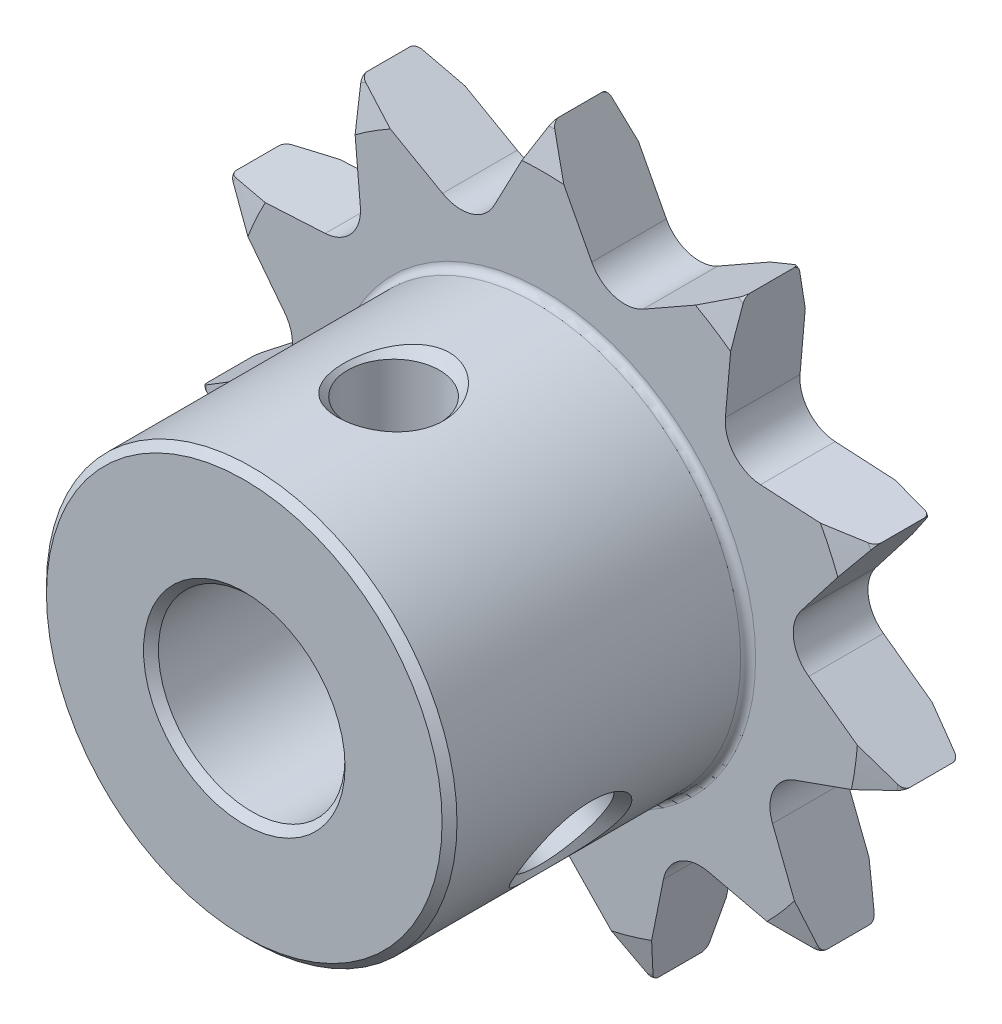
from build123d import *

# Parameters (mm, degrees)
SKETCH_2_W          = 302.005499825
SKETCH_2_H          = 246.129864536
CUT_EXTRUDE_1_DEPTH = 2


with BuildPart() as part:
    # 草图1 → 旋转1 (revolve)
    with BuildSketch(Plane(origin=(0, 0, 0), x_dir=(0, 0, -1), z_dir=(1, 0, 0)), mode=Mode.PRIVATE) as revolve_1_sk:
        with BuildLine():
            Line((-10, 2.7), (-9.8, 2.5))
            Line((-9.8, 2.5), (-0.2, 2.5))
            Line((-0.2, 2.5), (0, 2.7))
            Line((0, 2.7), (0, 8.45))
            Line((0, 8.45), (-0.241626884, 9.351763809))
            ThreePointArc((-0.241626884, 9.351763809), (-0.313059764, 9.458670668), (-0.43481205, 9.5))
            Line((-0.43481205, 9.5), (-1.56518795, 9.5))
            ThreePointArc((-1.56518795, 9.5), (-1.686940236, 9.458670668), (-1.758373116, 9.351763809))
            Line((-1.758373116, 9.351763809), (-2, 8.45))
            Line((-2, 8.45), (-2, 5.7))
            ThreePointArc((-2, 5.7), (-2.058578644, 5.558578644), (-2.2, 5.5))
            Line((-2.2, 5.5), (-9.8, 5.5))
            Line((-9.8, 5.5), (-10, 5.3))
            Line((-10, 5.3), (-10, 2.7))
        make_face()
    revolve(revolve_1_sk.sketch.rotate(Axis((0, 0, 0), (0, 0, 1)), 270), axis=Axis((0, 0, 0), (0, 0, 1)))

    # 草图2 → 切除-拉伸1 (cut)
    with BuildSketch(Plane.XY):
        with Locations((0.692673165, 3.694256879)):
            Rectangle(SKETCH_2_W, SKETCH_2_H)
        with BuildLine():
            Line((-9.403303698, -1.351990964), (-6.749929888, -2.292665419))
            ThreePointArc((-6.749929888, -2.292665419), (-6.174441043, -2.819772743), (-6.152944955, -3.59988008))
            Line((-6.152944955, -3.59988008), (-7.179620956, -6.221176972))
            Line((-7.179620956, -6.221176972), (-4.438893858, -5.578000496))
            ThreePointArc((-4.438893858, -5.578000496), (-3.6697861, -5.710298635), (-3.229944571, -6.354945026))
            Line((-3.229944571, -6.354945026), (-2.67645929, -9.115183249))
            Line((-2.67645929, -9.115183249), (-0.718540392, -7.092359827))
            ThreePointArc((-0.718540392, -7.092359827), (0, -6.787845057), (0.718540392, -7.092359827))
            Line((0.718540392, -7.092359827), (2.67645929, -9.115183249))
            Line((2.67645929, -9.115183249), (3.229944571, -6.354945026))
            ThreePointArc((3.229944571, -6.354945026), (3.6697861, -5.710298635), (4.438893858, -5.578000496))
            Line((4.438893858, -5.578000496), (7.179620956, -6.221176972))
            Line((7.179620956, -6.221176972), (6.152944955, -3.59988008))
            ThreePointArc((6.152944955, -3.59988008), (6.174441043, -2.819772743), (6.749929888, -2.292665419))
            Line((6.749929888, -2.292665419), (9.403303698, -1.351990964))
            Line((9.403303698, -1.351990964), (7.12242879, 0.298121355))
            ThreePointArc((7.12242879, 0.298121355), (6.718754582, 0.966011072), (6.917910871, 1.720574729))
            Line((6.917910871, 1.720574729), (8.641503956, 3.946442624))
            Line((8.641503956, 3.946442624), (5.830591809, 4.101471366))
            ThreePointArc((5.830591809, 4.101471366), (5.129911013, 4.445093196), (4.889504032, 5.187544557))
            Line((4.889504032, 5.187544557), (5.136087766, 7.991908562))
            Line((5.136087766, 7.991908562), (2.687583126, 6.602633199))
            ThreePointArc((2.687583126, 6.602633199), (1.912356943, 6.512889638), (1.308714211, 7.007505642))
            Line((1.308714211, 7.007505642), (0, 9.5))
            Line((0, 9.5), (-1.308714211, 7.007505642))
            ThreePointArc((-1.308714211, 7.007505642), (-1.912356943, 6.512889638), (-2.687583126, 6.602633199))
            Line((-2.687583126, 6.602633199), (-5.136087766, 7.991908562))
            Line((-5.136087766, 7.991908562), (-4.889504032, 5.187544557))
            ThreePointArc((-4.889504032, 5.187544557), (-5.129911013, 4.445093196), (-5.830591809, 4.101471366))
            Line((-5.830591809, 4.101471366), (-8.641503956, 3.946442624))
            Line((-8.641503956, 3.946442624), (-6.917910871, 1.720574729))
            ThreePointArc((-6.917910871, 1.720574729), (-6.718754582, 0.966011072), (-7.12242879, 0.298121355))
            Line((-7.12242879, 0.298121355), (-9.403303698, -1.351990964))
        make_face(mode=Mode.SUBTRACT)
    extrude(amount=CUT_EXTRUDE_1_DEPTH, mode=Mode.SUBTRACT)

    # 草图3 → 切除-旋转1 (revolve, cut)
    with BuildSketch(Plane.XY.offset(6), mode=Mode.PRIVATE) as cut_revolve_1_sk:
        Polygon((0, 0), (-1.5, 0), (-1.5, 2.5), (-1.2295, 2.7705), (-1.2295, 5.2295), (-1.5, 5.5), (-1.5, 8), (0, 8), align=None)
    revolve(cut_revolve_1_sk.sketch.rotate(Axis((0, 5.5, 6), (0, -1, 0)), 180), axis=Axis((0, 5.5, 6), (0, -1, 0)), mode=Mode.SUBTRACT)

    # 草图4 → 切除-旋转2 (revolve, cut)
    with BuildSketch(Plane.XY.offset(6), mode=Mode.PRIVATE) as cut_revolve_2_sk:
        Polygon((0, 0), (0.75, 1.299038106), (2.915063509, 0.049038106), (3.014073381, -0.320471766), (5.143629849, -1.549971766), (5.513139721, -1.450961894), (7.67820323, -2.700961894), (6.92820323, -4), align=None)
    revolve(cut_revolve_2_sk.sketch.rotate(Axis((4.763139721, -2.75, 6), (-0.8660254037844383, 0.5000000000000009, 0)), 180), axis=Axis((4.763139721, -2.75, 6), (-0.8660254037844383, 0.5000000000000009, 0)), mode=Mode.SUBTRACT)


solid = part.part
